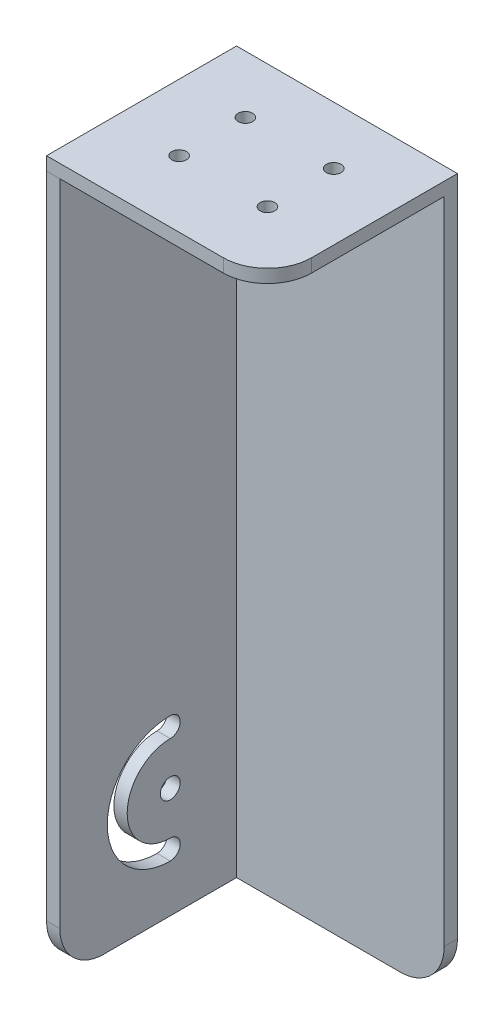
SolidWorks part; units mm, degrees
ref_plane "前视基准面" through (0, 0, 0) normal (0, 0, 1) x (1, 0, 0)
ref_plane "上视基准面" through (0, 0, 0) normal (0, 1, 0) x (1, 0, 0)
ref_plane "右视基准面" through (0, 0, 0) normal (1, 0, 0) x (0, 0, -1)
sketch "草图1" plane through (0, 0, 0) normal (0, 0, 1) x (1, 0, 0)
  line L1 (-25, 80) -> (25, 80)
  line L2 (-25, 80) -> (-25, -80)
  line L3 (-25, -80) -> (25, -80)
  line L4 (25, 80) -> (25, -80)
  line L5 (-25, 80) -> (25, -80) construction
  line L6 (-25, -80) -> (25, 80) construction
  point P0 (0, 0)
  dimension "D1" = 50
  dimension "D2" = 160
extrude "凸台-拉伸1" add sketch "草图1" along normal blind 3
sketch "草图2" plane through (0, 0, 3) normal (0, 0, 1) x (1, 0, 0)
  line L0 (25, -80) -> (25, 80) construction
  line L1 (-25, 80) -> (25, 80)
  line L2 (-25, 80) -> (-25, 77)
  line L3 (-25, 77) -> (25, 77)
  line L4 (25, 80) -> (25, 77)
  dimension "D1" = 3
extrude "凸台-拉伸2" add sketch "草图2" along normal blind 40
sketch "草图5" plane through (-25, 0, 0) normal (-1, 0, 0) x (0, 0, 1)
  line L0 (3, -80) -> (0, -80) construction
  line L1 (3, 77) -> (43, 77)
  line L2 (3, 77) -> (3, -80)
  line L3 (3, -80) -> (43, -80)
  line L4 (43, 77) -> (43, -80)
  line L5 (43, 80) -> (43, 77) construction
extrude "凸台-拉伸3" add sketch "草图5" against normal blind 3 separate body
sketch "草图6" plane through (-22, 0, 0) normal (1, 0, 0) x (0, 0, -1)
  line L0 (-3, -80) -> (-43, -80) construction
  line L1 (-43, -80) -> (-43, 77) construction
  circle A0 centre (-18, -55) radius 2.25
  circle A1 centre (-18, -55) radius 12 construction
  arc A2 (-18, -40.75) -> (-18, -69.25) centre (-18, -55) ccw
  arc A3 (-18, -45.25) -> (-18, -64.75) centre (-18, -55) ccw
  arc A4 (-18, -45.25) -> (-18, -40.75) centre (-18, -43) ccw
  arc A5 (-18, -69.25) -> (-18, -64.75) centre (-18, -67) ccw
  dimension "D1" = 4.5
  dimension "D3" = 2.25
  dimension "D2" = 12
  dimension "D4" = 25
  dimension "D5" = 25
extrude "切除-拉伸1" cut sketch "草图6" against normal blind 10
hole_wizard "M4 螺纹孔1" positions "草图7" profile "草图8" tap size "M4" standard "ISO" end condition through all
sketch "草图7" plane through (0, 80, 0) normal (0, 1, 0) x (1, 0, 0)
  line L0 (0, 0) -> (0, -43) construction
  line L1 (25, -43) -> (-25, -43) construction
  point P0 (-10, -13)
  point P2 (10, -13)
  point P14 (-10, -28)
  point P16 (10, -28)
  dimension "D1" = 20
  dimension "D2" = 30
  dimension "D3" = 15
sketch "草图8" plane through (-10, 80, 13) normal (1, 0, 0) x (0, 0, 1)
  line L0 (0, 0) -> (0, 160)
  line L1 (0, 160) -> (1.65, 160)
  line L2 (1.65, 160) -> (1.65, 0)
  line L5 (1.65, 0) -> (0, 0)
  line L11 (0, -6.35) -> (0, 107.95) construction
  dimension "通孔螺纹孔钻头直径" = 3.3
  dimension "通孔螺纹孔钻头深度" = 160
cosmetic thread "孔螺蚊线1" parameters "D2"=4
cosmetic thread "孔螺蚊线2" parameters "D2"=4
cosmetic thread "孔螺蚊线3" parameters "D2"=4
cosmetic thread "孔螺蚊线4" parameters "D2"=4
fillet "圆角1" radius 10 2 edges at (25, -80, 1.5) (25, 78.5, 43)
fillet "圆角2" radius 10 1 edges at (-23.5, -80, 43)
